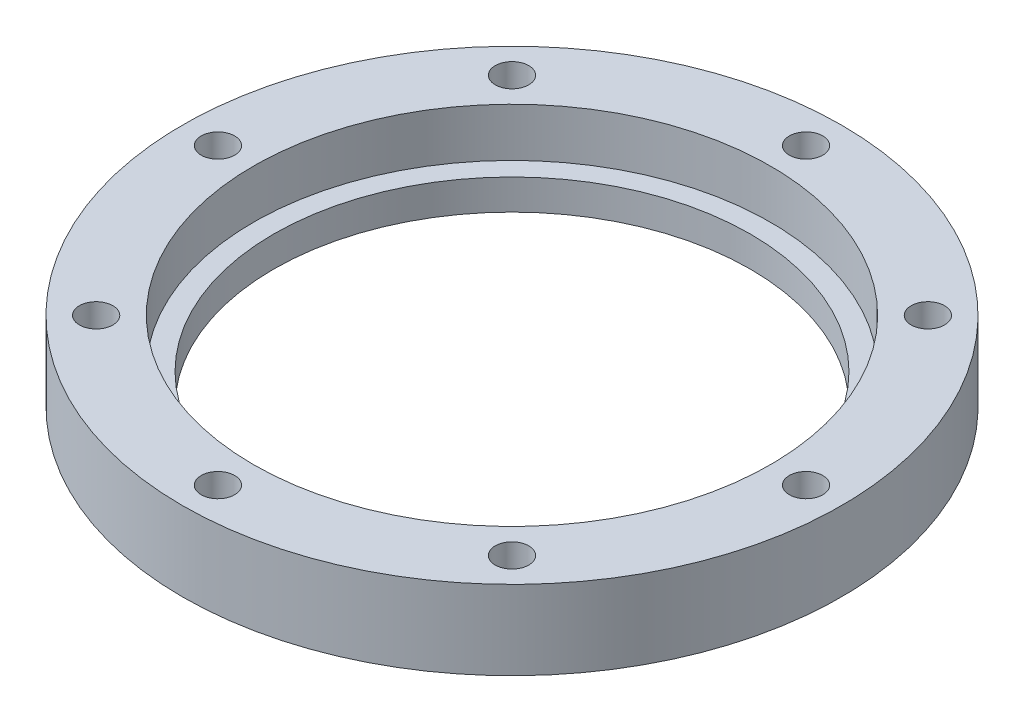
from build123d import *

# Parameters (mm, degrees)
SKETCH_1_R         = 32.5
SKETCH_1_R_2       = 23.5
EXTRUDE_1_DEPTH    = 3
SKETCH_2_R         = 32.5
SKETCH_2_R_2       = 25.5
EXTRUDE_2_DEPTH    = 4.8
HOLE_WIZARD_M4_1_D = 3.3


with BuildPart() as part:
    # 草图1 → 凸台-拉伸1 (new body)
    with BuildSketch(Plane(origin=(0, 0, 0), x_dir=(1, 0, 0), z_dir=(0, 1, 0))):
        with Locations(Location((0, 0, 0), (0, 0, 270))):
            Circle(SKETCH_1_R)
        with Locations(Location((0, 0, 0), (0, 0, 270))):
            Circle(SKETCH_1_R_2, mode=Mode.SUBTRACT)
    extrude(amount=EXTRUDE_1_DEPTH)

    # 草图2 → 凸台-拉伸2 (add)
    with BuildSketch(Plane(origin=(0, 3, 0), x_dir=(1, 0, 0), z_dir=(0, 1, 0))):
        with Locations(Location((0, 0, 0), (0, 0, 270))):
            Circle(SKETCH_2_R)
        with Locations(Location((0, 0, 0), (0, 0, 270))):
            Circle(SKETCH_2_R_2, mode=Mode.SUBTRACT)
    extrude(amount=EXTRUDE_2_DEPTH)

    # M4 螺纹孔1 (through all)
    with Locations(Plane(origin=(0, 7.8, 0), x_dir=(1, 0, 0), z_dir=(0, 1, 0))):
        with Locations((0, 29), (20.506096654, 20.506096654), (29, 0), (20.506096654, -20.506096654), (0, -29), (-20.506096654, -20.506096654), (-29, 0), (-20.506096654, 20.506096654), (0, 0)):
            Hole(HOLE_WIZARD_M4_1_D / 2)


solid = part.part
